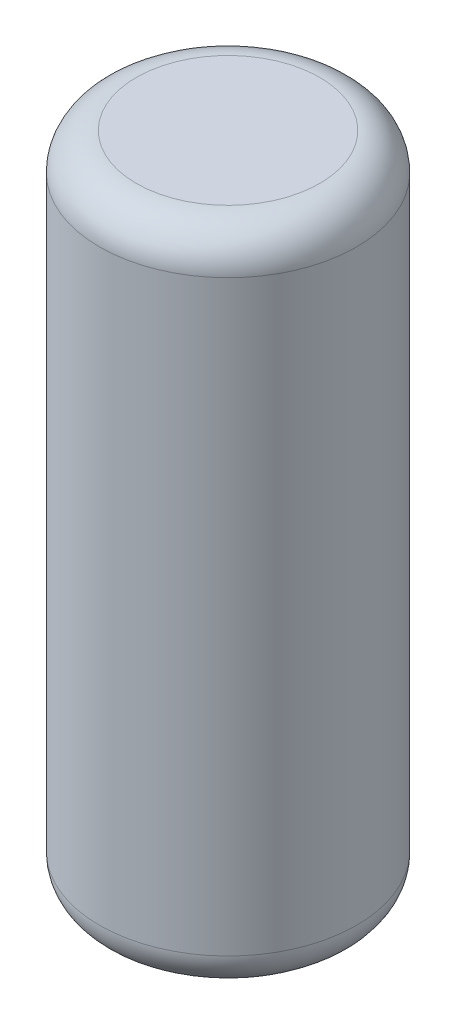
from build123d import *

# Parameters (mm, degrees)
SKETCH1_R           = 3.5
BOSS_EXTRUDE1_DEPTH = 18
FILLET1_R           = 1


with BuildPart() as part:
    # Sketch1 → Boss-Extrude1 (new body)
    with BuildSketch(Plane(origin=(0, 0, 0), x_dir=(1, 0, 0), z_dir=(0, 1, 0))):
        with Locations(Location((0, 0, 0), (0, 0, 270))):
            Circle(SKETCH1_R)
    extrude(amount=BOSS_EXTRUDE1_DEPTH)

    # Fillet1
    fillet1_edges = [part.edges().sort_by_distance(p)[0] for p in [
        (0, 0, -3.5),
        (0, 18, -3.5),
    ]]
    fillet(fillet1_edges, radius=FILLET1_R)


solid = part.part
